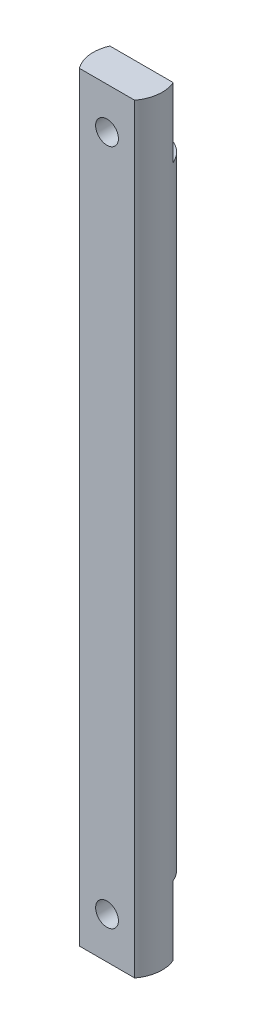
SolidWorks part; units mm, degrees
ref_plane "Front Plane" through (0, 0, 0) normal (0, 0, 1) x (1, 0, 0)
ref_plane "Top Plane" through (0, 0, 0) normal (0, 1, 0) x (1, 0, 0)
ref_plane "Right Plane" through (0, 0, 0) normal (1, 0, 0) x (0, 0, -1)
other "Configuration Table"
sketch "Sketch1" plane through (0, 0, 0) normal (0, 1, 0) x (1, 0, 0)
  circle A0 centre (0, 0) radius 5
  dimension "D1" = 10
extrude "Boss-Extrude1" add sketch "Sketch1" along normal blind 110
sketch "Sketch2" plane through (0, 110, 0) normal (0, 1, 0) x (1, 0, 0)
  line L0 (-4, -3) -> (4, -3)
  line L1 (0, 5) -> (0, -5) construction
  circle A0 centre (0, 0) radius 5 construction
  arc A2 (-4, -3) -> (4, -3) centre (0, 0) ccw
  dimension "D1" = 3
extrude "Cut-Extrude1" cut sketch "Sketch2" against normal through all
sketch "Sketch3" plane through (0, 110, 0) normal (0, 1, 0) x (1, 0, 0)
  line L0 (-4.5826, 2) -> (4.5826, 2)
  circle A0 centre (0, 0) radius 5 construction
  arc A1 (4.5826, 2) -> (-4.5826, 2) centre (0, 0) ccw
  point P5 (0, 2)
  dimension "D1" = 2
extrude "Cut-Extrude2" cut sketch "Sketch3" against normal blind 10
ref_plane "Plane1" through (0, 55, 0) normal (0, 1, 0) x (1, 0, 0)
mirror "Mirror1" about plane through (0, 55, 0) normal (0, 1, 0) of "Cut-Extrude2"
sketch "Sketch4" plane through (0, 0, -2) normal (0, 0, -1) x (-1, 0, 0)
  line L0 (4.5826, 110) -> (-4.5826, 110) construction
  line L1 (4.5826, 0) -> (-4.5826, 0) construction
  point P0 (0, 104)
  point P4 (0, 110)
  point P5 (0, 6)
  dimension "D1" = 6
  dimension "D2" = 6
hole_wizard "M4 Tapped Hole2" positions "Sketch4" profile "Sketch5" tap size "M4" standard "GB" end condition through all
sketch "Sketch5" plane through (0, 104, -2) normal (1, 0, 0) x (0, 1, 0)
  line L0 (0, 0) -> (0, 5)
  line L1 (0, 5) -> (1.65, 5)
  line L2 (1.65, 5) -> (1.65, 0)
  line L5 (1.65, 0) -> (0, 0)
  line L11 (0, -6.35) -> (0, 107.95) construction
  dimension "通孔螺纹孔钻头直径" = 3.3
  dimension "通孔螺纹孔钻头深度" = 5
cosmetic thread "Cosmetic thread 3" parameters "D2"=4
cosmetic thread "Cosmetic thread 4" parameters "D2"=4
